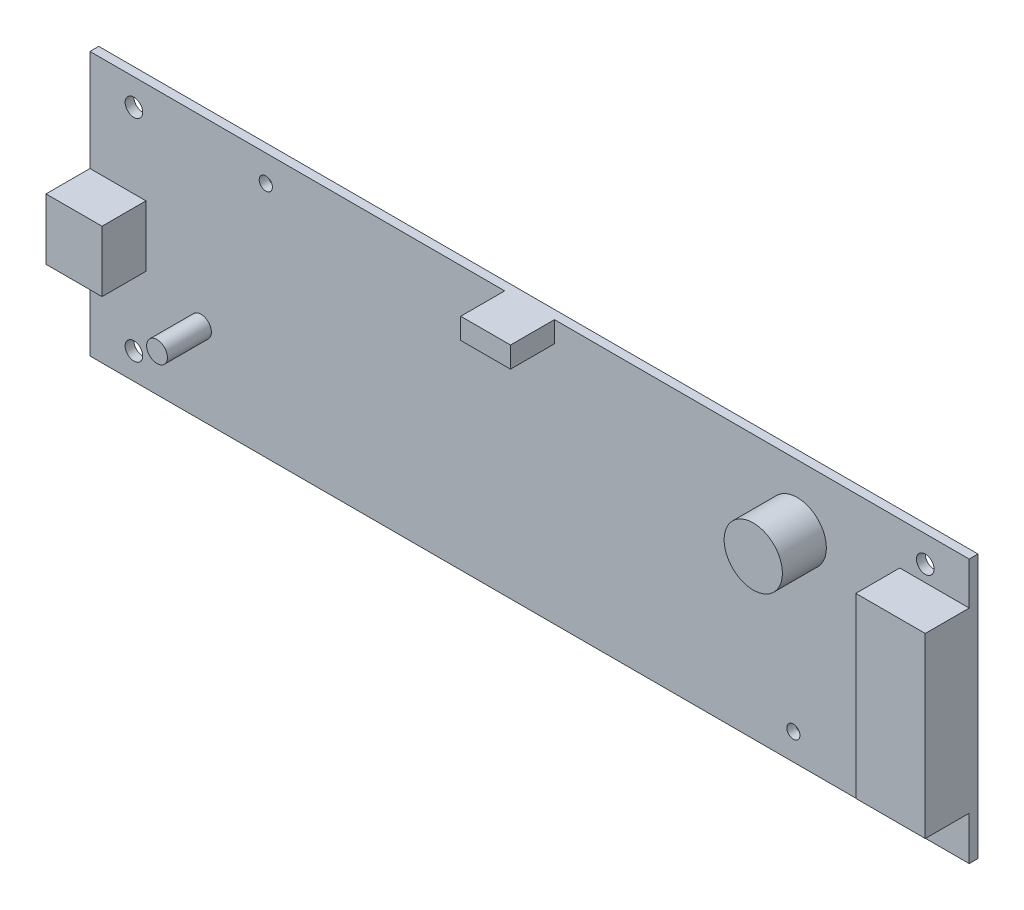
SolidWorks part; units mm, degrees
ref_plane "Front Plane" through (0, 0, 0) normal (0, 0, 1) x (1, 0, 0)
ref_plane "Top Plane" through (0, 0, 0) normal (0, 1, 0) x (1, 0, 0)
ref_plane "Right Plane" through (0, 0, 0) normal (1, 0, 0) x (0, 0, -1)
other "Configuration Table"
sketch "Sketch1" plane through (0, 0, 0) normal (0, 0, 1) x (1, 0, 0)
  line L1 (-50, 15) -> (50, 15)
  line L2 (-50, 15) -> (-50, -15)
  line L3 (-50, -15) -> (50, -15)
  line L4 (50, 15) -> (50, -15)
  line L5 (-50, 15) -> (50, -15) construction
  line L6 (-50, -15) -> (50, 15) construction
  line L7 (-45, 12) -> (45, 12) construction
  line L8 (-45, 12) -> (-45, -12) construction
  line L9 (-45, -12) -> (45, -12) construction
  line L10 (45, 12) -> (45, -12) construction
  line L11 (-45, 12) -> (45, -12) construction
  line L12 (-45, -12) -> (45, 12) construction
  circle A0 centre (-45, -12) radius 1
  circle A1 centre (-45, 12) radius 1
  circle A2 centre (45, 12) radius 1
  circle A3 centre (45, -12) radius 1
  point P0 (0, 0)
  point P6 (0, 0)
  dimension "D5" = 2
  dimension "D1" = 100
  dimension "D2" = 30
  dimension "D3" = 24
  dimension "D4" = 90
extrude "Boss-Extrude1" add sketch "Sketch1" along normal blind 1
sketch "Sketch2" plane through (0, 0, 1) normal (0, 0, 1) x (1, 0, 0)
  line L0 (50, -15) -> (50, 15) construction
  line L1 (42.1029, 10.1733) -> (50, 10.1733)
  line L2 (42.1029, 10.1733) -> (42.1029, -10.0282)
  line L3 (42.1029, -10.0282) -> (50, -10.0282)
  line L4 (50, 10.1733) -> (50, -10.0282)
  line L5 (42.1029, 10.1733) -> (50, -10.0282) construction
  line L6 (42.1029, -10.0282) -> (50, 10.1733) construction
  line L7 (50, 15) -> (-50, 15) construction
  line L8 (-2.8295, 12.6173) -> (2.8295, 12.6173)
  line L9 (-2.8295, 12.6173) -> (-2.8295, 15)
  line L10 (-2.8295, 15) -> (2.8295, 15)
  line L11 (2.8295, 12.6173) -> (2.8295, 15)
  line L12 (-2.8295, 12.6173) -> (2.8295, 15) construction
  line L13 (-2.8295, 15) -> (2.8295, 12.6173) construction
  line L14 (-50, 15) -> (-50, -15) construction
  line L15 (-43.6289, -3.4697) -> (-50, -3.4697)
  line L16 (-43.6289, -3.4697) -> (-43.6289, 3.4697)
  line L17 (-43.6289, 3.4697) -> (-50, 3.4697)
  line L18 (-50, -3.4697) -> (-50, 3.4697)
  line L19 (-43.6289, -3.4697) -> (-50, 3.4697) construction
  line L20 (-43.6289, 3.4697) -> (-50, -3.4697) construction
  circle A0 centre (30.4404, 7.9743) radius 3.3121
  circle A1 centre (-37.3722, -5.7496) radius 1.1827
  point P0 (46.0515, 0.0726)
  point P9 (-46.8145, 0)
  point P10 (0, 13.8087)
extrude "Boss-Extrude2" add sketch "Sketch2" along normal blind 5
sketch "Sketch3" plane through (0, 0, 0) normal (0, 0, -1) x (-1, 0, 0)
  line L0 (-50, -7) -> (50, -7) construction
  line L1 (-50, -15) -> (-50, 15) construction
  line L2 (50, 15) -> (50, -15) construction
  line L3 (0, 0) -> (0, 15) construction
  line L4 (-15, -4.5) -> (-10, -4.5)
  line L5 (-15, -4.5) -> (-15, -9.5)
  line L6 (-15, -9.5) -> (-10, -9.5)
  line L7 (-10, -4.5) -> (-10, -9.5)
  line L8 (-15, -4.5) -> (-10, -9.5) construction
  line L9 (-15, -9.5) -> (-10, -4.5) construction
  line L10 (-40, -4.5) -> (-35, -4.5)
  line L11 (-40, -4.5) -> (-40, -9.5)
  line L12 (-40, -9.5) -> (-35, -9.5)
  line L13 (-35, -4.5) -> (-35, -9.5)
  line L14 (-40, -4.5) -> (-35, -9.5) construction
  line L15 (-40, -9.5) -> (-35, -4.5) construction
  line L16 (-50, 15) -> (50, 15) construction
  line L17 (50, -15) -> (-50, -15) construction
  line L18 (40, -4.5) -> (35, -4.5)
  line L19 (40, -4.5) -> (40, -9.5)
  line L20 (40, -9.5) -> (35, -9.5)
  line L21 (35, -4.5) -> (35, -9.5)
  line L22 (15, -4.5) -> (15, -9.5)
  line L23 (15, -4.5) -> (10, -4.5)
  line L24 (10, -4.5) -> (10, -9.5)
  line L25 (15, -9.5) -> (10, -9.5)
  point P6 (-12.5, -7)
  point P11 (-37.5, -7)
  dimension "D1" = 5
  dimension "D2" = 5
  dimension "D3" = 5
  dimension "D4" = 5
  dimension "D5" = 25
  dimension "D6" = 12.5
  dimension "D7" = 8
extrude "Boss-Extrude3" add sketch "Sketch3" along normal blind 1
sketch "Sketch4" plane through (0, 0, -1) normal (0, 0, -1) x (-1, 0, 0)
  circle A0 centre (-37.5, -7) radius 1
  circle A1 centre (-12.5, -7) radius 1
  circle A2 centre (12.5, -7) radius 1
  circle A3 centre (37.5, -7) radius 1
  dimension "D1" = 2
extrude "Boss-Extrude4" add sketch "Sketch4" along normal blind 1
sketch "Sketch5" plane through (0, 0, 1) normal (0, 0, 1) x (1, 0, 0)
  line L0 (-45, 12) -> (-20.9389, 12) construction
  line L1 (45, -12) -> (21.7858, -12) construction
  circle A0 centre (30, -12) radius 0.75
  circle A1 centre (-30, 12) radius 0.75
  circle A2 centre (-45, 12) radius 1 construction
  circle A3 centre (45, -12) radius 1 construction
  dimension "D1" = 1.5
  dimension "D2" = 15
  dimension "D3" = 1.5
  dimension "D4" = 15
extrude "Cut-Extrude1" cut sketch "Sketch5" against normal blind 10
